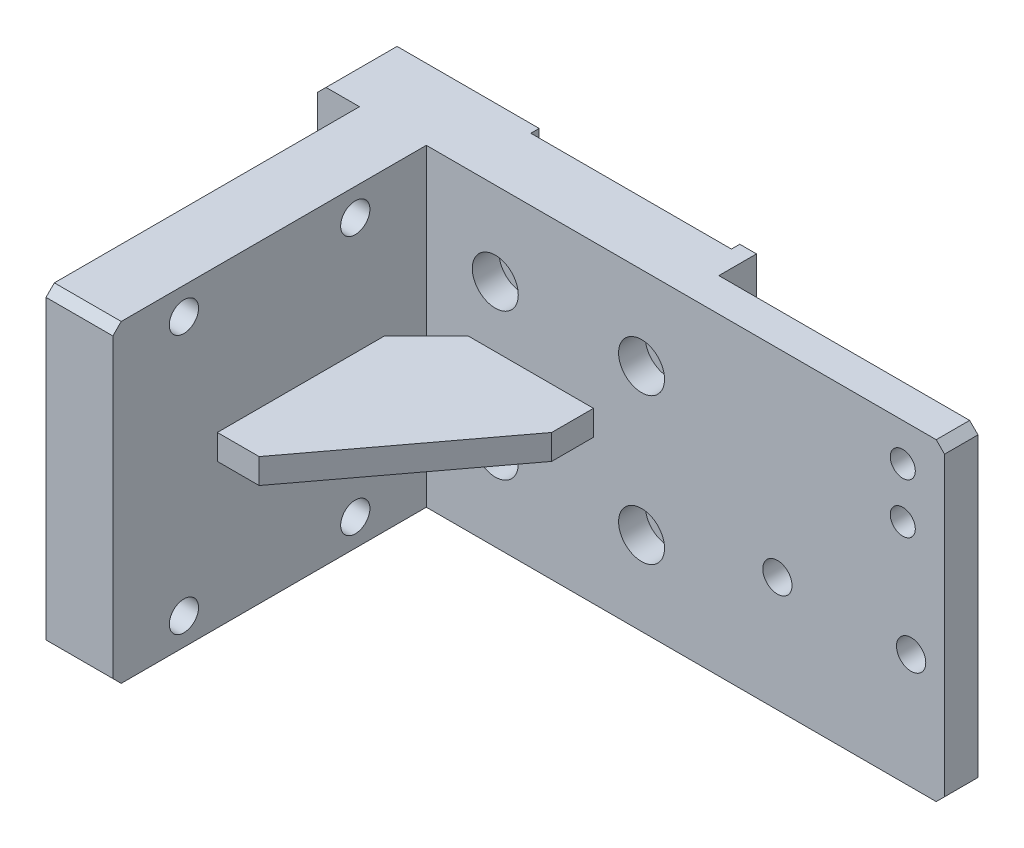
from build123d import *

# Parameters (mm, degrees)
SKETCH_1_W                   = 150
SKETCH_1_H                   = 75
EXTRUDE_1_DEPTH              = 17
HOLE_WIZARD_M6_1_D           = 6.6
HOLE_WIZARD_M6_1_CBORE_D     = 11
HOLE_WIZARD_M6_1_CBORE_DEPTH = 6.4
SKETCH_8_W                   = 16
SKETCH_8_H                   = 75
EXTRUDE_2_DEPTH              = 75
HOLE_WIZARD_7_0_7_1_D        = 7
SKETCH_11_W                  = 48
SKETCH_11_H                  = 2
CUT_EXTRUDE_1_DEPTH          = 141.406552554
EXTRUDE_3_DEPTH              = 3
CHAMFER_1_SIZE               = 2
SKETCH_13_W                  = 62
SKETCH_13_H                  = 9
CUT_EXTRUDE_2_DEPTH          = 141.406552554
HOLE_WIZARD_7_0_7_2_D        = 7
HOLE_WIZARD_6_0_6_1_D        = 6


with BuildPart() as part:
    # 草图1 → 凸台-拉伸1 (new body)
    with BuildSketch(Plane.XY):
        Rectangle(SKETCH_1_W, SKETCH_1_H)
    extrude(amount=EXTRUDE_1_DEPTH)

    # M6 六角凹头螺钉的柱形沉头孔1 (through all)
    with Locations(Plane.XY.offset(17)):
        with Locations((2.5, 17.5), (-32.5, 17.5), (-32.5, -17.5), (2.5, -17.5)):
            CounterBoreHole(HOLE_WIZARD_M6_1_D / 2, HOLE_WIZARD_M6_1_CBORE_D / 2, HOLE_WIZARD_M6_1_CBORE_DEPTH)

    # 草图8 → 凸台-拉伸2 (add)
    with BuildSketch(Plane.XY.offset(17)):
        with Locations((-57, 0)):
            Rectangle(SKETCH_8_W, SKETCH_8_H)
    extrude(amount=EXTRUDE_2_DEPTH)

    # Ø7.0 (7) 直径孔1 (through all)
    with Locations(Plane(origin=(-49, 0, 0), x_dir=(0, 0, -1), z_dir=(1, 0, 0))):
        with Locations((-75, 31), (-75, -31), (-34, -31), (-34, 31)):
            Hole(HOLE_WIZARD_7_0_7_1_D / 2)

    # 草图11 → 切除-拉伸1 (cut, through all)
    with BuildSketch(Plane.XZ.offset(37.5)):
        with Locations((-15, 1)):
            Rectangle(SKETCH_11_W, SKETCH_11_H)
    extrude(amount=-CUT_EXTRUDE_1_DEPTH, mode=Mode.SUBTRACT)

    # 草图12 → 凸台-拉伸3 (add, symmetric)
    with BuildSketch(Plane(origin=(0, 0, 0), x_dir=(1, 0, 0), z_dir=(0, 1, 0))):
        Polygon((-49, -67), (-39, -67), (-9, -27), (-9, -17), (-39, -17), (-49, -27), align=None)
    extrude(amount=EXTRUDE_3_DEPTH, both=True)

    # 倒角1
    chamfer_1_edges = [part.edges().sort_by_distance(p)[0] for p in [
        (75, -37.5, 8.5),
        (75, 37.5, 8.5),
        (-57, -37.5, 92),
        (-57, 37.5, 92),
        (-75, 37.5, 8.5),
        (-75, -37.5, 8.5),
    ]]
    chamfer(chamfer_1_edges, length=CHAMFER_1_SIZE)

    # 草图13 → 切除-拉伸2 (cut, through all)
    with BuildSketch(Plane.XZ.offset(37.5)):
        with Locations((44, 4.5)):
            Rectangle(SKETCH_13_W, SKETCH_13_H)
    extrude(amount=-CUT_EXTRUDE_2_DEPTH, mode=Mode.SUBTRACT)

    # Ø7.0 (7) 直径孔2 (through all)
    with Locations(Plane.XY.offset(17)):
        with Locations((35, -10), (67, -10)):
            Hole(HOLE_WIZARD_7_0_7_2_D / 2)

    # Ø6.0 (6) 直径孔1 (through all)
    with Locations(Plane.XY.offset(17)):
        with Locations((65, 28.5), (65, 16.5)):
            Hole(HOLE_WIZARD_6_0_6_1_D / 2)


solid = part.part
